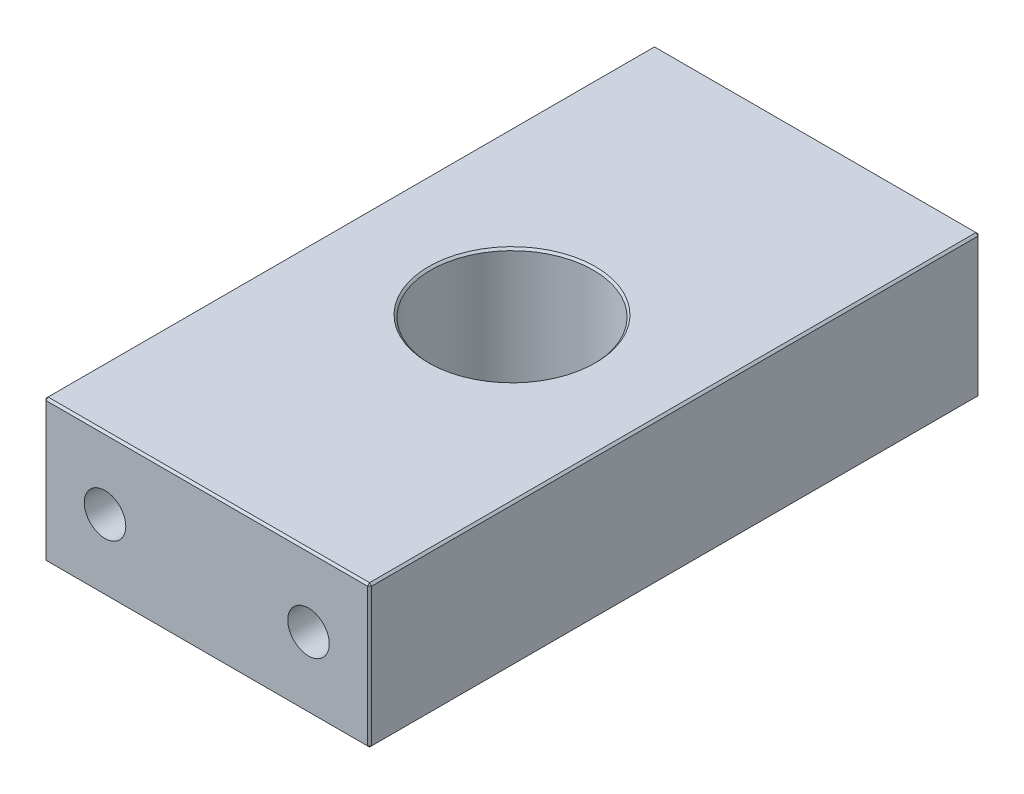
SolidWorks part; units mm, degrees
material "合金钢"
ref_plane "前视基准面" through (0, 0, 0) normal (0, 0, 1) x (1, 0, 0)
ref_plane "上视基准面" through (0, 0, 0) normal (0, 1, 0) x (1, 0, 0)
ref_plane "右视基准面" through (0, 0, 0) normal (1, 0, 0) x (0, 0, -1)
sketch "草图1" plane through (0, 0, 0) normal (0, 1, 0) x (1, 0, 0)
  line L1 (-40, -75) -> (40, -75)
  line L2 (-40, -75) -> (-40, 75)
  line L3 (-40, 75) -> (40, 75)
  line L4 (40, -75) -> (40, 75)
  line L5 (-40, -75) -> (40, 75) construction
  line L6 (-40, 75) -> (40, -75) construction
  circle A0 centre (0, 0) radius 20
  point P0 (0, 0)
  dimension "D3" = 40
  dimension "D1" = 80
  dimension "D2" = 150
extrude "凸台-拉伸1" add sketch "草图1" along normal blind 35
chamfer "倒角1" distance 0.5 angle 45 14 edges at (40, 17.5, -75) (-40, 17.5, -75) (-40, 17.5, 75) (0, 35, 75) (-40, 35, 0) (0, 35, -75) (40, 35, 0) (40, 17.5, 75) (0, 0, 75) (-40, 0, 0) (0, 0, -75) (40, 0, 0) (0, 0, 20) (0, 35, 20)
hole_wizard "M12 螺纹孔1" positions "草图2" profile "草图3" tap size "M12" standard "GB"
sketch "草图2" plane through (0, 0, 75) normal (0, 0, 1) x (1, 0, 0)
  line L1 (40, 34.5) -> (40, 0.5) construction
  line L2 (-40, 0.5) -> (-40, 34.5) construction
  point P0 (25, 17.5)
  point P2 (-25, 17.5)
  point P13 (40, 17.5)
  dimension "D1" = 15
  dimension "D2" = 15
sketch "草图3" plane through (25, 17.5, 75) normal (1, 0, 0) x (0, -1, 0)
  line L0 (0, 0) -> (0, 32.3144)
  line L1 (0, 32.3144) -> (5.1, 29.25)
  line L2 (5.1, 29.25) -> (5.1, 0)
  line L5 (5.1, 0) -> (0, 0)
  line L10 (0, 32.3144) -> (-5.1, 29.25) construction
  line L11 (0, -6.35) -> (0, 107.95) construction
  dimension "螺纹孔钻头直径" = 10.2
  dimension "螺纹孔钻头深度" = 29.25
  dimension "导头角度" = 118
cosmetic thread "孔螺蚊线1"
cosmetic thread "孔螺蚊线2"
hole_wizard "M12 螺纹孔2" positions "草图4" profile "草图5" tap size "M12" standard "GB"
sketch "草图4" plane through (0, 0, -75) normal (0, 0, -1) x (-1, 0, 0)
  line L0 (39.5, 0.5) -> (39.5, 34.5) construction
  line L1 (39.5, 34.5) -> (-39.5, 34.5) construction
  point P0 (-25, 17.5)
  point P2 (25, 17.5)
  dimension "D1" = 14.5
  dimension "D2" = 64.5
  dimension "D3" = 17
sketch "草图5" plane through (25, 17.5, -75) normal (1, 0, 0) x (0, 1, 0)
  line L0 (0, 0) -> (0, 32.3144)
  line L1 (0, 32.3144) -> (5.1, 29.25)
  line L2 (5.1, 29.25) -> (5.1, 0)
  line L5 (5.1, 0) -> (0, 0)
  line L10 (0, 32.3144) -> (-5.1, 29.25) construction
  line L11 (0, -6.35) -> (0, 107.95) construction
  dimension "螺纹孔钻头直径" = 10.2
  dimension "螺纹孔钻头深度" = 29.25
  dimension "导头角度" = 118
cosmetic thread "孔螺蚊线3" parameters "D1"=24, "D2"=12
cosmetic thread "孔螺蚊线4" parameters "D1"=24, "D2"=12
